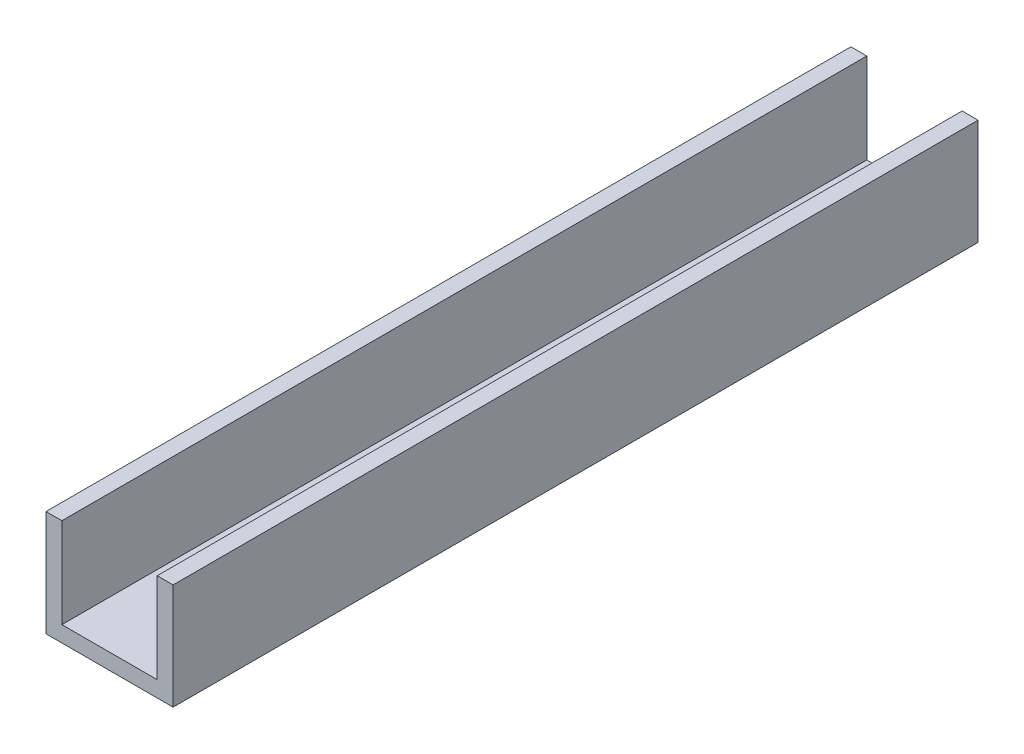
from build123d import *

# Parameters (mm, degrees)
EXTRUDE_1_DEPTH     = 45
SKETCH_2_W          = 15
SKETCH_2_H          = 12
CUT_EXTRUDE_1_DEPTH = 10


with BuildPart() as part:
    # 草图1 → 凸台-拉伸1 (new, symmetric)
    with BuildSketch(Plane.XY):
        Polygon((-6, -5), (6, -5), (6, 5), (4.5, 5), (4.5, -3.5), (-4.5, -3.5), (-4.5, 5), (-6, 5), align=None)
    extrude(amount=EXTRUDE_1_DEPTH, both=True)

    # 草图2 → 切除-拉伸1 (cut, symmetric)
    with BuildSketch(Plane(origin=(0, 0, 0), x_dir=(0, 0, -1), z_dir=(1, 0, 0))):
        with Locations((-38.5, 0)):
            Rectangle(SKETCH_2_W, SKETCH_2_H)
    extrude(amount=CUT_EXTRUDE_1_DEPTH, both=True, mode=Mode.SUBTRACT)


solid = part.part
